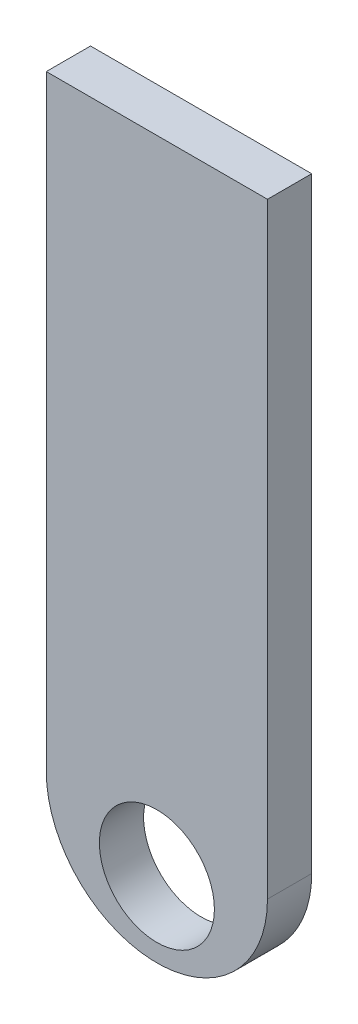
SolidWorks part; units mm, degrees
material "AISI 1045 钢，冷拔"
ref_plane "Front Plane" through (0, 0, 0) normal (0, 0, 1) x (1, 0, 0)
ref_plane "Top Plane" through (0, 0, 0) normal (0, 1, 0) x (1, 0, 0)
ref_plane "Right Plane" through (0, 0, 0) normal (1, 0, 0) x (0, 0, -1)
sketch "Sketch1" plane through (0, 0, 0) normal (0, 0, 1) x (1, 0, 0)
  line L0 (-25, 0) -> (-25, 137)
  line L1 (-25, 137) -> (25, 137)
  line L2 (25, 137) -> (25, 0)
  arc A0 (-25, 0) -> (25, 0) centre (0, 0) ccw
  dimension "D2" = 50
  dimension "D3" = 137
extrude "Boss-Extrude1" add sketch "Sketch1" along normal blind 10
sketch "Sketch2" plane through (0, 0, 10) normal (0, 0, 1) x (1, 0, 0)
  circle A0 centre (0, -8) radius 13
  arc A1 (-25, 0) -> (25, 0) centre (0, 0) ccw construction
  dimension "D1" = 26
  dimension "D2" = 8
extrude "Cut-Extrude1" cut sketch "Sketch2" against normal through all
